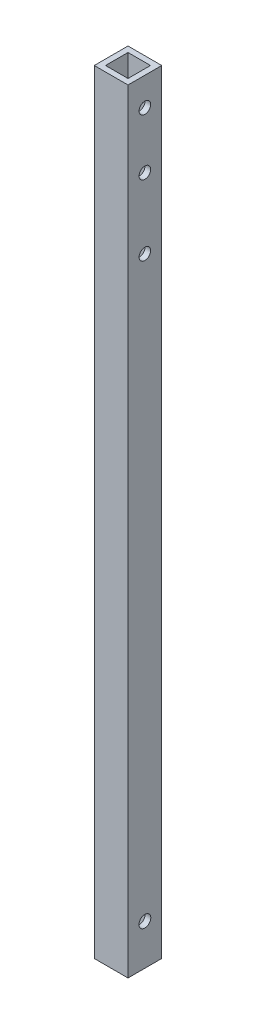
from build123d import *

# Parameters (mm, degrees)
SKETCH_1_W          = 12
SKETCH_1_H          = 12
SKETCH_1_W_2        = 8
SKETCH_1_H_2        = 8
EXTRUDE_1_DEPTH     = 275
SKETCH_3_R          = 2.05
SKETCH_3_R_2        = 2.1
CUT_EXTRUDE_2_DEPTH = 276.327078218


with BuildPart() as part:
    # 草图1 → 凸台-拉伸1 (new body)
    with BuildSketch(Plane(origin=(0, 0, 0), x_dir=(1, 0, 0), z_dir=(0, 1, 0))):
        Rectangle(SKETCH_1_W, SKETCH_1_H)
        Rectangle(SKETCH_1_W_2, SKETCH_1_H_2, mode=Mode.SUBTRACT)
    extrude(amount=EXTRUDE_1_DEPTH)

    # 草图3 → 切除-拉伸2 (cut, through all)
    with BuildSketch(Plane.ZY.offset(6)):
        with Locations((0, 265)):
            Circle(SKETCH_3_R)
        with Locations((0, 245)):
            Circle(SKETCH_3_R)
        with Locations((0, 220)):
            Circle(SKETCH_3_R)
        with Locations((0, 14.5)):
            Circle(SKETCH_3_R_2)
    extrude(amount=-CUT_EXTRUDE_2_DEPTH, mode=Mode.SUBTRACT)


solid = part.part
